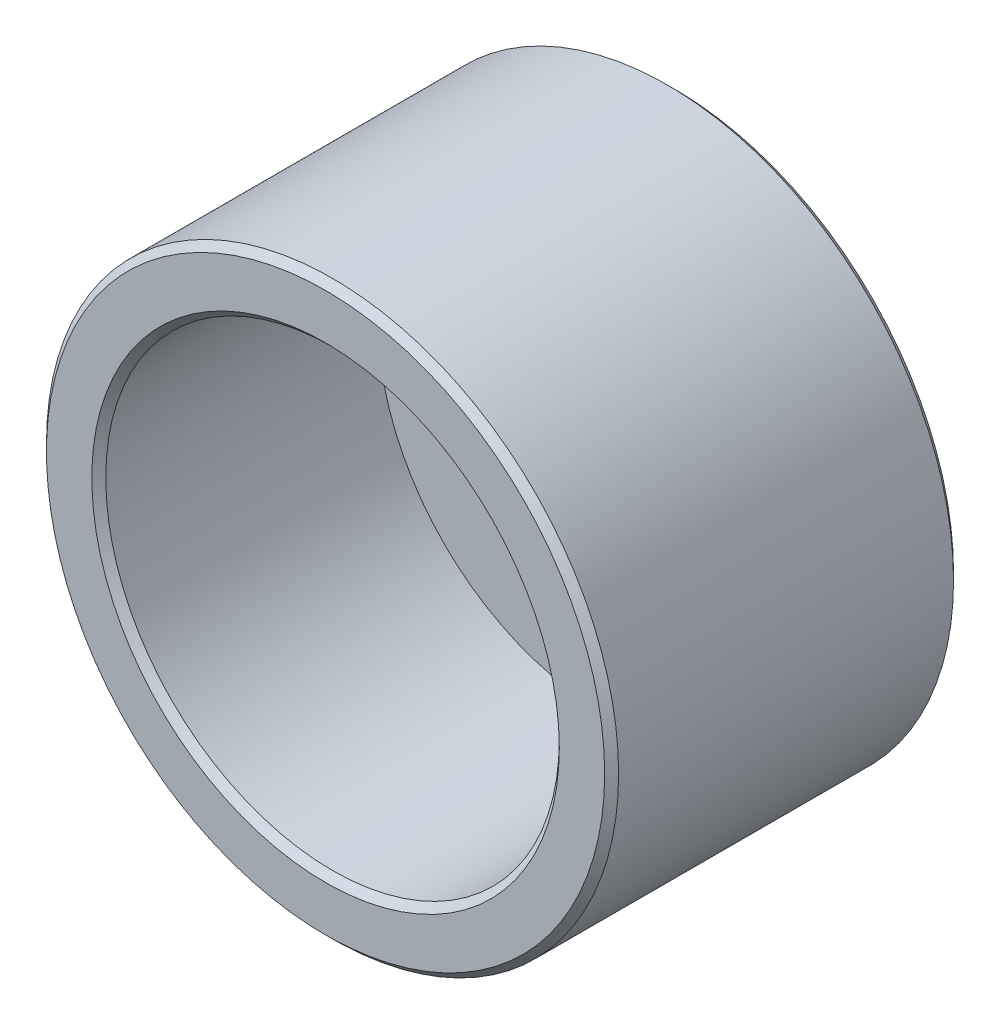
SolidWorks part; units mm, degrees
material "Q235-A"
ref_plane "Front Plane" through (0, 0, 0) normal (0, 0, 1) x (1, 0, 0)
ref_plane "Top Plane" through (0, 0, 0) normal (0, 1, 0) x (1, 0, 0)
ref_plane "Right Plane" through (0, 0, 0) normal (1, 0, 0) x (0, 0, -1)
sketch "Sketch1" plane through (0, 0, 0) normal (0, 0, 1) x (1, 0, 0)
  circle A1 centre (0, 0) radius 20.5
  dimension "D2" = 41
extrude "Boss-Extrude1" add sketch "Sketch1" along normal blind 25
chamfer "Chamfer1" distance 0.5 angle 45 2 edges at (20.5, 0, 25) (20.5, 0, 0)
sketch "Sketch5" plane through (0, 0, 25) normal (0, 0, 1) x (1, 0, 0)
  circle A0 centre (0, 0) radius 16.25
  dimension "D1" = 32.5
extrude "Cut-Extrude1" cut sketch "Sketch5" against normal blind 20
chamfer "Chamfer2" distance 0.5 angle 45 1 edges at (16.25, 0, 25)
sketch "Sketch6" plane through (0, 0, 0) normal (0, 0, -1) x (-1, 0, 0)
  circle A0 centre (0, 0) radius 10.5
  dimension "D1" = 21
extrude "Cut-Extrude2" cut sketch "Sketch6" against normal blind 31
